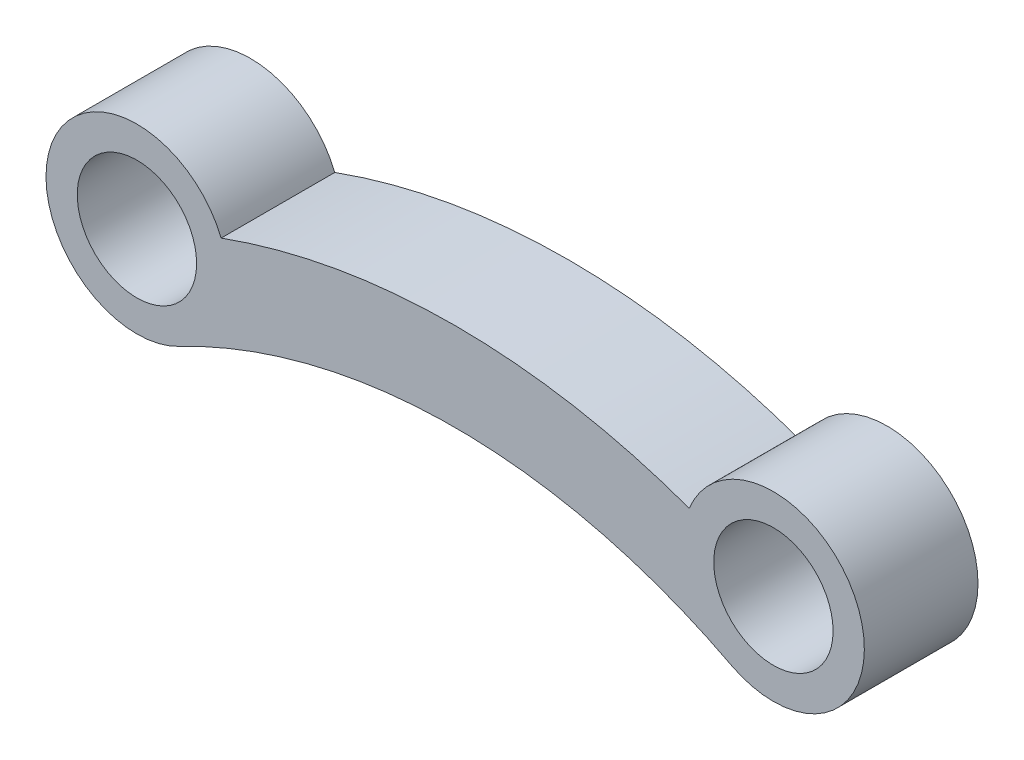
SolidWorks part; units mm, degrees
ref_plane "Front Plane" through (0, 0, 0) normal (0, 0, 1) x (1, 0, 0)
ref_plane "Top Plane" through (0, 0, 0) normal (0, 1, 0) x (1, 0, 0)
ref_plane "Right Plane" through (0, 0, 0) normal (1, 0, 0) x (0, 0, -1)
other "Configuration Table"
sketch "Sketch1" plane through (0, 0, 0) normal (0, 0, 1) x (1, 0, 0)
  line L1 (-14, -25.3) -> (-14, -23.8) construction
  line L2 (-14, -25.3) -> (-14, -26.8) construction
  arc A1 (-26.7382, 2.1582) -> (-25.5154, -0.2767) centre (-28, 0) ccw
  arc A2 (-2.4846, -0.2767) -> (-1.2618, 2.1582) centre (0, 0) ccw
  arc A3 (-14, 5.1152) -> (-1.2618, 2.1582) centre (-14, -23.8) cw
  arc A4 (-14, 5.1152) -> (-26.7382, 2.1582) centre (-14, -23.8) ccw
  arc A5 (-14, 2.1152) -> (-25.5154, -0.2767) centre (-14, -26.8) ccw
  arc A6 (-14, 2.1152) -> (-2.4846, -0.2767) centre (-14, -26.8) cw
extrude "Boss-Extrude1" add sketch "Sketch1" along normal blind 5
sketch "Sketch2" plane through (0, 0, 5) normal (0, 0, 1) x (1, 0, 0)
  circle A0 centre (-28, 0) radius 1.5
  circle A1 centre (0, 0) radius 1.5
extrude "Cut-Extrude1" cut sketch "Sketch2" against normal blind 3
sketch "Sketch3" plane through (0, 0, 5) normal (0, 0, 1) x (1, 0, 0)
  arc A0 (-27.059, 3.8877) -> (-24.149, -1.0816) centre (-28, 0) ccw
  arc A1 (-3.851, -1.0816) -> (-0.941, 3.8877) centre (0, 0) ccw
  arc A2 (-24.149, -1.0816) -> (-3.851, -1.0816) centre (-14, -26.8) cw
  arc A3 (-25.5349, 4.5566) -> (-0.941, 3.8877) centre (-14, -23.8) cw
  arc A4 (-25.5349, 4.5566) -> (-27.059, 3.8877) centre (-14, -23.8) ccw
extrude "Boss-Extrude2" add sketch "Sketch3" against normal through all
sketch "Sketch4" plane through (0, 0, 5) normal (0, 0, 1) x (1, 0, 0)
  circle A0 centre (-28, 0) radius 2.625
  circle A1 centre (0, 0) radius 2.625
extrude "Cut-Extrude2" cut sketch "Sketch4" against normal through all
sketch "Sketch5" plane through (0, 0, 5) normal (0, 0, 1) x (1, 0, 0)
  line L0 (-27.059, 3.8877) -> (-14.206, 10.7407)
  line L1 (-14.206, 10.7407) -> (-0.941, 3.8877)
  arc A0 (-26.1479, -3.5454) -> (-1.8521, -3.5454) centre (-14, -26.8) cw
  arc A1 (-27.059, 3.8877) -> (-24.149, -1.0816) centre (-28, 0) ccw construction
  arc A2 (-3.851, -1.0816) -> (-0.941, 3.8877) centre (0, 0) ccw construction
  arc A3 (-25.5766, 1.0088) -> (-2.4234, 1.0088) centre (-14, -26.8) cw
  circle A4 centre (-28, 0) radius 2.625 construction
  circle A5 centre (0, 0) radius 2.625 construction
  circle A6 centre (-28, 0) radius 4
  circle A7 centre (0, 0) radius 4
  arc M5 (-0.941, 3.8877) -> (-27.059, 3.8877) centre (-14, -23.8) ccw
extrude "Cut-Extrude3" cut sketch "Sketch5" against normal through all contours L1 L0 M5 | A7 A6 A3 M5
sketch "Sketch7" plane through (0, 0, 5) normal (0, 0, 1) x (1, 0, 0)
  line L0 (-26.1479, -3.5454) -> (-24.1778, 0.2781)
  line L1 (-24.1778, 0.2781) -> (-14.7566, 2.143)
  line L2 (-14.7566, 2.143) -> (-4.3423, 0.2781)
  line L3 (-4.3423, 0.2781) -> (-2.5365, -2.3155)
  line L4 (-2.5365, -2.3155) -> (-1.8521, -3.5454)
  arc A0 (-26.1479, -3.5454) -> (-1.8521, -3.5454) centre (-14, -26.8) cw
  arc A1 (-24.2952, 1.5082) -> (-24.149, -1.0816) centre (-28, 0) ccw construction
  arc A2 (-3.851, -1.0816) -> (-3.7048, 1.5082) centre (0, 0) ccw construction
extrude "Boss-Extrude3" add sketch "Sketch7" against normal through all
